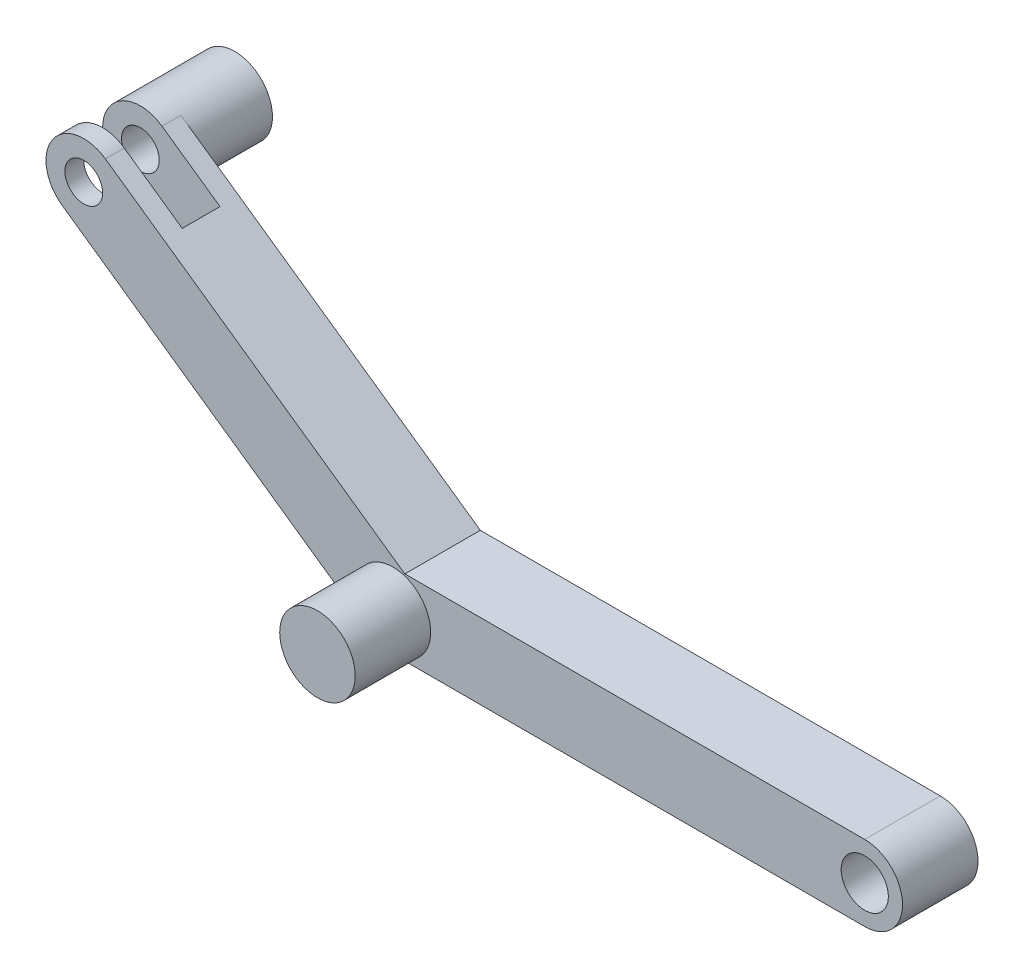
SolidWorks part; units mm, degrees
ref_plane "Front Plane" through (0, 0, 0) normal (0, 0, 1) x (1, 0, 0)
ref_plane "Top Plane" through (0, 0, 0) normal (0, 1, 0) x (1, 0, 0)
ref_plane "Right Plane" through (0, 0, 0) normal (1, 0, 0) x (0, 0, -1)
sketch "Sketch1" plane through (0, 0, 0) normal (0, 0, 1) x (1, 0, 0)
  line L0 (0, 0) -> (-100, 0) construction
  line L1 (-100, 0) -> (-165.5322, 45.8861) construction
  line L2 (0, 8) -> (-97.4776, 8)
  line L3 (-97.4776, 8) -> (-160.9436, 52.4393)
  line L4 (0, -8) -> (-102.5224, -8)
  line L5 (-102.5224, -8) -> (-170.1208, 39.3329)
  arc A0 (0, 8) -> (0, -8) centre (0, 0) cw
  arc A1 (-160.9436, 52.4393) -> (-170.1208, 39.3329) centre (-165.5322, 45.8861) ccw
  dimension "D1" = 100
  dimension "D2" = 80
  dimension "D3" = 145
  dimension "D4" = 8
  dimension "D5" = 8
extrude "Boss-Extrude1" add sketch "Sketch1" along normal blind 16
sketch "Sketch2" plane through (0, 0, 16) normal (0, 0, 1) x (1, 0, 0)
  line L0 (0, 0) -> (-54.9552, 0) construction
  line L1 (-12.72, 2.1626) -> (-27.0921, -18.363) construction
  circle A0 centre (0, 0) radius 5
  point P10 (-14.2342, 0)
  dimension "D1" = 10
  dimension "D3" = 25.057
  dimension "D4" = 55
  dimension "D5" = 11.66
extrude "Cut-Extrude1" cut sketch "Sketch2" against normal blind 16
sketch "Sketch3" plane through (0, 0, 0) normal (0, 0, -1) x (-1, 0, 0)
  line L0 (97.4776, 8) -> (102.5224, -8) construction
  circle A1 centre (100, 0) radius 8
extrude "Boss-Extrude2" add sketch "Sketch3" against normal blind 32
sketch "Sketch4" plane through (0, 0, 16) normal (0, 0, 1) x (1, 0, 0)
  circle A0 centre (-165.5322, 45.8861) radius 8
extrude "Boss-Extrude3" add sketch "Sketch4" against normal blind 32
sketch "Sketch5" plane through (-37.4876, -53.5378, 0) normal (-0.5736, -0.8192, 0) x (0.8192, -0.5736, 0)
  line L0 (-161.9152, 16) -> (-161.9152, 0) construction
  line L1 (-146.9152, 4) -> (-176.9152, 4)
  line L2 (-146.9152, 4) -> (-146.9152, 12)
  line L3 (-146.9152, 12) -> (-176.9152, 12)
  line L4 (-176.9152, 4) -> (-176.9152, 12)
  line L5 (-146.9152, 4) -> (-176.9152, 12) construction
  line L6 (-146.9152, 12) -> (-176.9152, 4) construction
  point P0 (-161.9152, 8)
  dimension "D1" = 8
  dimension "D2" = 30
extrude "Cut-Extrude2" cut sketch "Sketch5" against normal blind 38
sketch "Sketch6" plane through (0, 0, 16) normal (0, 0, 1) x (1, 0, 0)
  circle A0 centre (-165.5322, 45.8861) radius 4
  dimension "D1" = 8
extrude "Cut-Extrude3" cut sketch "Sketch6" against normal blind 38
